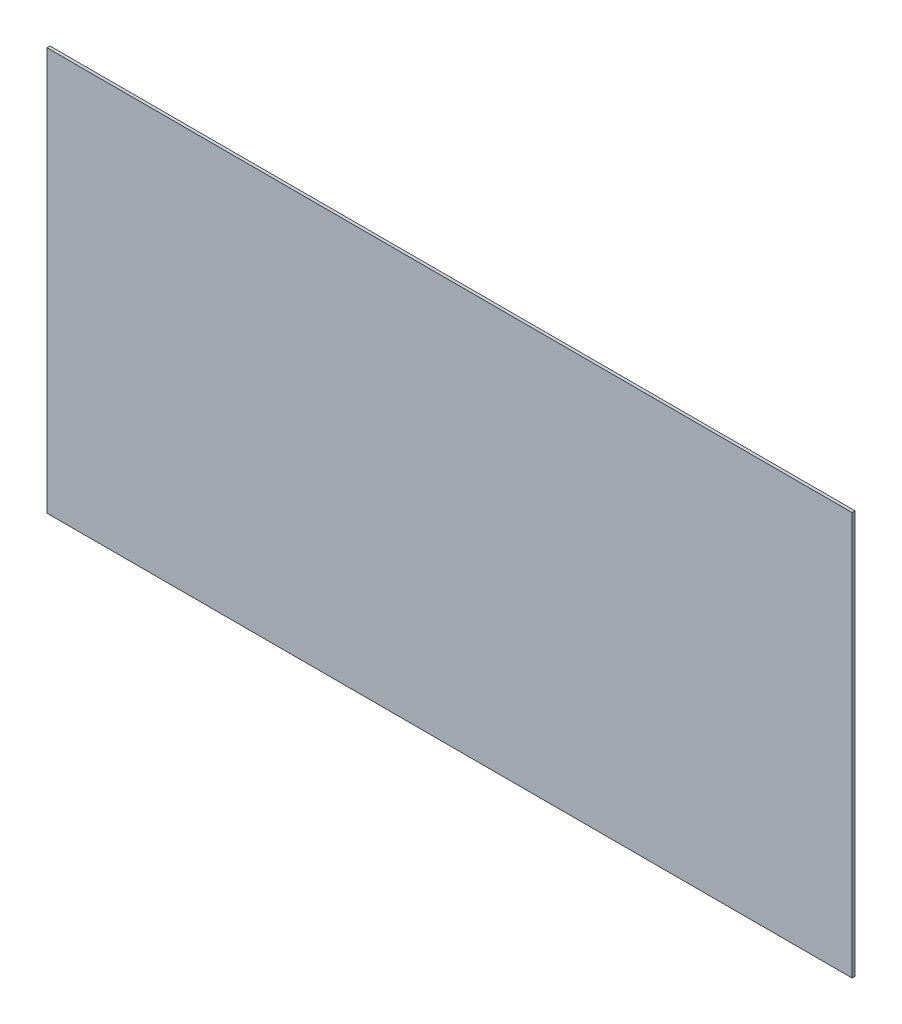
SolidWorks part; units mm, degrees
material "PMMA(有机玻璃)"
ref_plane "前视" through (0, 0, 0) normal (0, 0, 1) x (1, 0, 0)
ref_plane "上视" through (0, 0, 0) normal (0, 1, 0) x (1, 0, 0)
ref_plane "右视" through (0, 0, 0) normal (1, 0, 0) x (0, 0, -1)
sketch "草图1" plane through (0, 0, 0) normal (0, 0, 1) x (1, 0, 0)
  line L1 (-675, 338) -> (675, 338)
  line L2 (-675, 338) -> (-675, -338)
  line L3 (-675, -338) -> (675, -338)
  line L4 (675, 338) -> (675, -338)
  line L5 (-675, 338) -> (675, -338) construction
  line L6 (-675, -338) -> (675, 338) construction
  point P0 (0, 0)
  dimension "D1" = 676
  dimension "D2" = 1350
extrude "凸台-拉伸1" add sketch "草图1" along normal blind 5
hole_wizard "M5 间隙孔1" positions "草图3" profile "草图2" hole size "M5" standard "GB"
sketch "草图3" plane through (0, 0, 5) normal (0, 0, 1) x (1, 0, 0)
  line L0 (-427.5, 273) -> (-427.5, -273) construction
  line L1 (-427.5, -273) -> (427.5, -273) construction
  line L2 (0, 273) -> (0, -273) construction
  line L3 (427.5, 273) -> (-427.5, 273) construction
  line L5 (-427.5, 0) -> (427.5, 0) construction
  line L6 (427.5, -273) -> (427.5, 273) construction
  point P0 (-375, -261)
  point P46 (415.5, 250)
  point P48 (-415.5, 250)
  point P58 (-125, -261)
  point P59 (125, -261)
  point P61 (-125, 261)
  point P62 (125, 261)
  point P64 (-375, 261)
  point P88 (375, -261)
  point P89 (375, 261)
  point P108 (415.5, 0)
  point P109 (-415.5, 0)
  point P110 (415.5, -250)
  point P111 (-415.5, -250)
  dimension "D1" = 12
  dimension "D2" = 12
  dimension "D5" = 3
  dimension "D3" = 12
  dimension "D6" = 4
  dimension "D4" = 2
sketch "草图2" plane through (-375, -261, 5) normal (1, 0, 0) x (0, -1, 0)
  line L0 (0, 0) -> (0, 5)
  line L1 (0, 5) -> (2.75, 5)
  line L2 (2.75, 5) -> (2.75, 0)
  line L5 (2.75, 0) -> (0, 0)
  line L11 (0, -6.35) -> (0, 107.95) construction
  dimension "通孔孔直径" = 5.5
  dimension "通孔孔深度" = 5
